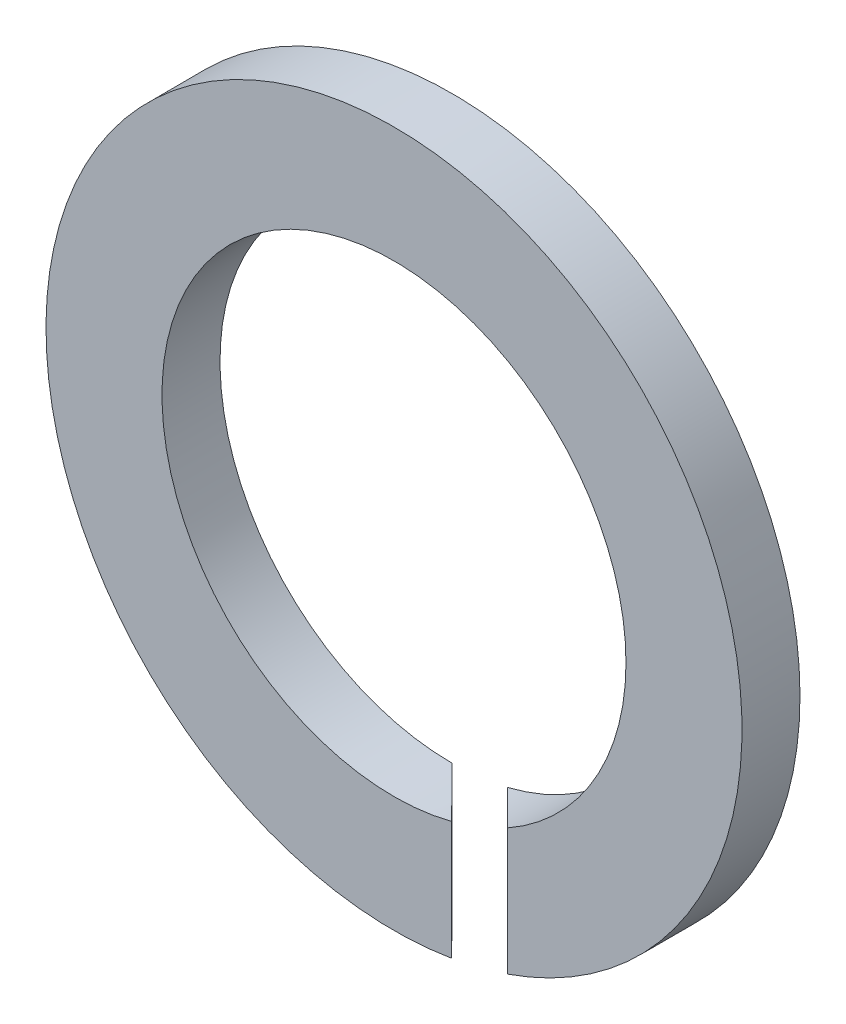
SolidWorks part; units mm, degrees
ref_plane "Front Plane" through (0, 0, 0) normal (0, 0, 1) x (1, 0, 0)
ref_plane "Top Plane" through (0, 0, 0) normal (0, 1, 0) x (1, 0, 0)
ref_plane "Right Plane" through (0, 0, 0) normal (1, 0, 0) x (0, 0, -1)
sketch "Sketch1" plane through (0, 0, 0) normal (0, 0, 1) x (1, 0, 0)
  circle A0 centre (0, 0) radius 4
  circle A1 centre (0, 0) radius 6
  dimension "D1" = 12
  dimension "D2" = 8
extrude "Boss-Extrude1" add sketch "Sketch1" along normal blind 1
sketch "Sketch2" plane through (0, 0, 0) normal (0, 1, 0) x (1, 0, 0)
  line L0 (0, 0) -> (0.959, 0)
  line L1 (6, 0) -> (-6, 0) construction
  line L2 (0.959, 0) -> (1.953, -1)
  line L3 (-6, -1) -> (6, -1) construction
  line L4 (1.953, -1) -> (0.994, -1)
  line L5 (0.994, -1) -> (0, 0)
  dimension "D1" = 1.41
extrude "Cut-Extrude1" cut sketch "Sketch2" against normal through all
